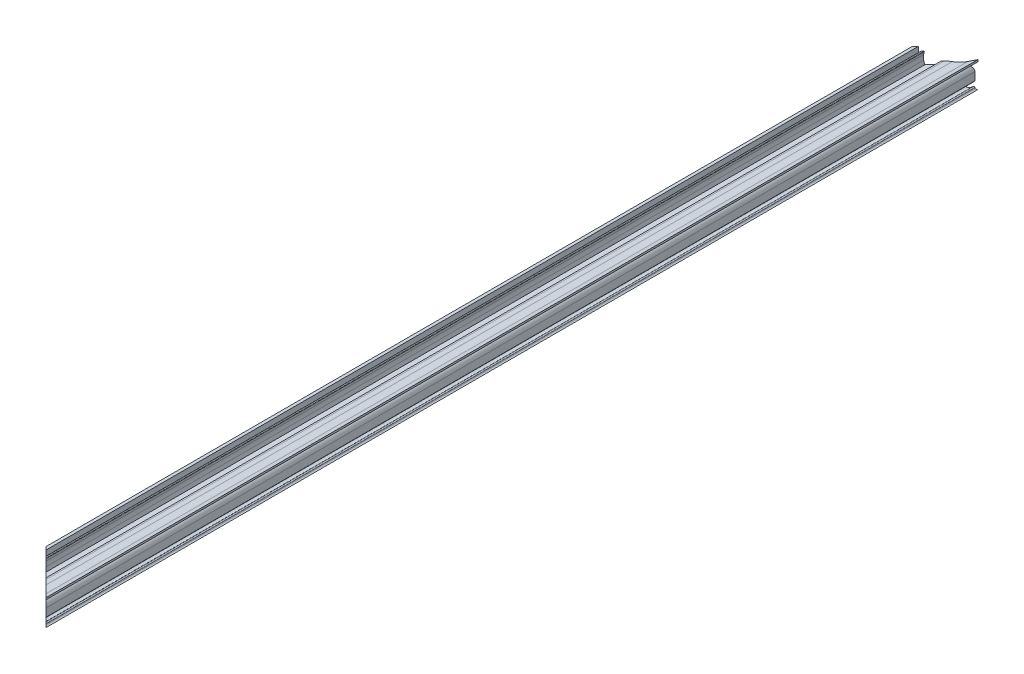
SolidWorks part; units mm, degrees
ref_plane "Front Plane" through (0, 0, 0) normal (0, 0, 1) x (1, 0, 0)
ref_plane "Top Plane" through (0, 0, 0) normal (0, 1, 0) x (1, 0, 0)
ref_plane "Right Plane" through (0, 0, 0) normal (1, 0, 0) x (0, 0, -1)
sketch "Sketch2" plane through (0, 0, 0) normal (0, 0, 1) x (1, 0, 0)
  line L0 (27.4296, 61.2035) -> (27.4296, 62.4835)
  line L1 (27.6297, 70.5806) -> (28.2239, 70.4974)
  line L2 (28.2521, 68.5355) -> (28.4794, 70.1587)
  line L3 (24.4296, 48.2035) -> (46.4296, 48.2035)
  line L4 (46.4296, 65.5674) -> (46.4296, 64.3068)
  line L5 (35.3196, 63.5648) -> (35.3196, 62.5671)
  line L6 (27.0637, 68.7019) -> (27.291, 70.3251)
  line L7 (28.6296, 62.5671) -> (34.1196, 62.5671)
  line L8 (24.4296, 73.2035) -> (26.4296, 73.2035)
  line L9 (43.408, 63.3348) -> (46.4296, 64.3068)
  line L10 (34.1196, 62.5671) -> (34.1196, 64.7671)
  line L11 (43.0405, 64.4771) -> (46.4296, 65.5674)
  line L13 (28.2521, 65.2634) -> (28.6296, 62.5671)
  line L14 (45.3996, 58.5671) -> (45.3996, 53.2529)
  line L15 (35.3196, 62.5671) -> (41.3996, 62.5671)
  line L16 (27.0637, 65.097) -> (27.4296, 62.4835)
  line L17 (34.1196, 64.7671) -> (35.1196, 64.7671)
  line L18 (24.4296, 48.2035) -> (24.4296, 73.2035)
  line L19 (26.4296, 73.2035) -> (26.4296, 61.2035)
  line L20 (26.4296, 61.2035) -> (27.4296, 61.2035)
  arc A0 (35.1196, 64.7671) -> (37.8501, 64.3871) centre (35.1196, 54.7671) cw
  arc A1 (28.4794, 70.1587) -> (28.2239, 70.4974) centre (28.1823, 70.2003) ccw
  arc A2 (37.8501, 64.3871) -> (43.0405, 64.4771) centre (40.2966, 73.0066) ccw
  arc A3 (27.0637, 65.097) -> (27.0637, 68.7019) centre (39.9382, 66.8995) cw
  arc A4 (27.291, 70.3251) -> (27.6297, 70.5806) centre (27.5881, 70.2835) cw
  arc A5 (37.5225, 63.2327) -> (43.408, 63.3348) centre (40.2966, 73.0066) ccw
  arc A6 (45.3996, 53.2529) -> (44.608, 52.8468) centre (44.8996, 53.2529) cw
  arc A7 (28.2521, 65.2634) -> (28.2521, 68.5355) centre (39.9382, 66.8995) cw
  arc A8 (44.608, 52.8468) -> (44.6629, 49.8013) centre (43.4996, 51.3035) ccw
  arc A9 (45.3996, 58.5671) -> (41.3996, 62.5671) centre (41.3996, 58.5671) ccw
  arc A10 (45.4401, 49.3477) -> (44.6629, 49.8013) centre (44.96, 49.4177) ccw
  arc A11 (35.3196, 63.5648) -> (37.5225, 63.2327) centre (35.1196, 54.7671) cw
  arc A12 (45.4401, 49.3477) -> (46.4296, 48.2035) centre (46.4296, 49.2035) ccw
  dimension "D7" = 4
  dimension "D9" = 3.8
  dimension "D10" = 2
  dimension "D4" = 0.3
  dimension "D5" = 0.3
  dimension "D12" = 0.5
  dimension "D3" = 1
  dimension "D11" = 3.1
extrude "Extrude1" add sketch "Sketch2" along normal blind 624
sketch "Sketch3" plane through (0, 48.2035, 0) normal (0, -1, 0) x (1, 0, 0)
  line L0 (46.4296, 624) -> (24.4296, 624)
  line L1 (24.4296, 624) -> (24.4296, 602)
  line L2 (24.4296, 624) -> (24.4296, 0) construction
  line L3 (24.4296, 602) -> (46.4296, 624)
  line L4 (46.4296, 0) -> (24.4296, 0)
  line L5 (24.4296, 0) -> (24.4296, 22)
  line L6 (24.4296, 22) -> (46.4296, 0)
  dimension "D1" = 22
  dimension "D2" = 22
extrude "Extrude2" cut sketch "Sketch3" against normal blind 30
